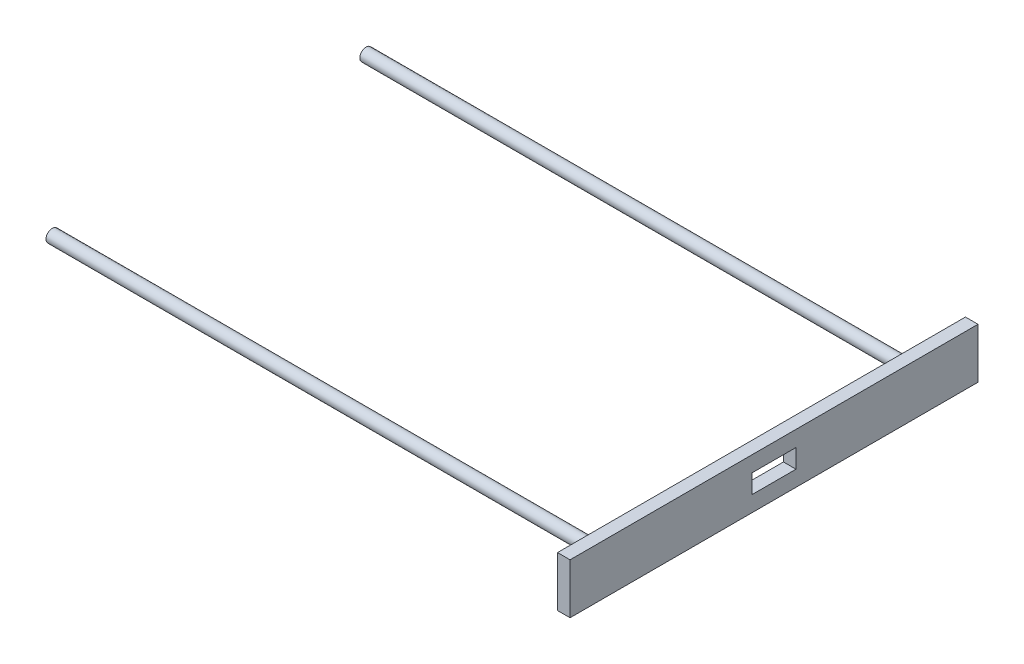
SolidWorks part; units mm, degrees
ref_plane "Front Plane" through (0, 0, 0) normal (0, 0, 1) x (1, 0, 0)
ref_plane "Top Plane" through (0, 0, 0) normal (0, 1, 0) x (1, 0, 0)
ref_plane "Right Plane" through (0, 0, 0) normal (1, 0, 0) x (0, 0, -1)
other "Configuration Table"
sketch "Sketch1" plane through (0, 0, 0) normal (1, 0, 0) x (0, 0, -1)
  line L0 (-330, 0) -> (330, 0) construction
  line L1 (-330, 45) -> (330, 45)
  line L2 (-330, 45) -> (-330, -45)
  line L3 (-330, -45) -> (330, -45)
  line L4 (330, 45) -> (330, -45)
  line L5 (-330, 45) -> (330, -45) construction
  line L6 (-330, -45) -> (330, 45) construction
  line L8 (-35, 15) -> (35, 15)
  line L9 (-35, 15) -> (-35, -15)
  line L10 (-35, -15) -> (35, -15)
  line L11 (35, 15) -> (35, -15)
  line L12 (-35, 15) -> (35, -15) construction
  line L13 (-35, -15) -> (35, 15) construction
  circle A0 centre (-250, 0) radius 10
  circle A1 centre (250, 0) radius 10
  point P0 (0, 0)
  point P12 (0, 0)
  dimension "D1" = 500
  dimension "D2" = 250
  dimension "D4" = 20
  dimension "D5" = 20
  dimension "D3" = 90
  dimension "D6" = 660
  dimension "D7" = 30
  dimension "D8" = 70
extrude "Boss-Extrude1" add sketch "Sketch1" along normal blind 20
sketch "Sketch2" plane through (20, 0, 0) normal (1, 0, 0) x (0, 0, -1)
  circle A0 centre (-250, 0) radius 10
  circle A1 centre (250, 0) radius 10
extrude "Boss-Extrude2" add sketch "Sketch2" against normal blind 900
sketch "Sketch3" plane through (20, 0, 0) normal (1, 0, 0) x (0, 0, -1)
  line L0 (330, 45) -> (-330, 45) construction
  line L1 (-325, -40) -> (325, -40)
  line L2 (-325, -40) -> (-325, 40)
  line L3 (-325, 40) -> (325, 40)
  line L4 (325, -40) -> (325, 40)
  line L5 (-325, -40) -> (325, 40) construction
  line L6 (-325, 40) -> (325, -40) construction
  line L7 (330, -45) -> (330, 45) construction
  line L9 (-451.8206, 117.8176) -> (451.8206, 117.8176)
  line L10 (-451.8206, 117.8176) -> (-451.8206, -117.8176)
  line L11 (-451.8206, -117.8176) -> (451.8206, -117.8176)
  line L12 (451.8206, 117.8176) -> (451.8206, -117.8176)
  line L13 (-451.8206, 117.8176) -> (451.8206, -117.8176) construction
  line L14 (-451.8206, -117.8176) -> (451.8206, 117.8176) construction
  point P0 (0, 0)
  point P10 (0, 0)
  dimension "D1" = 5
  dimension "D2" = 5
extrude "Cut-Extrude1" cut sketch "Sketch3" against normal through all
